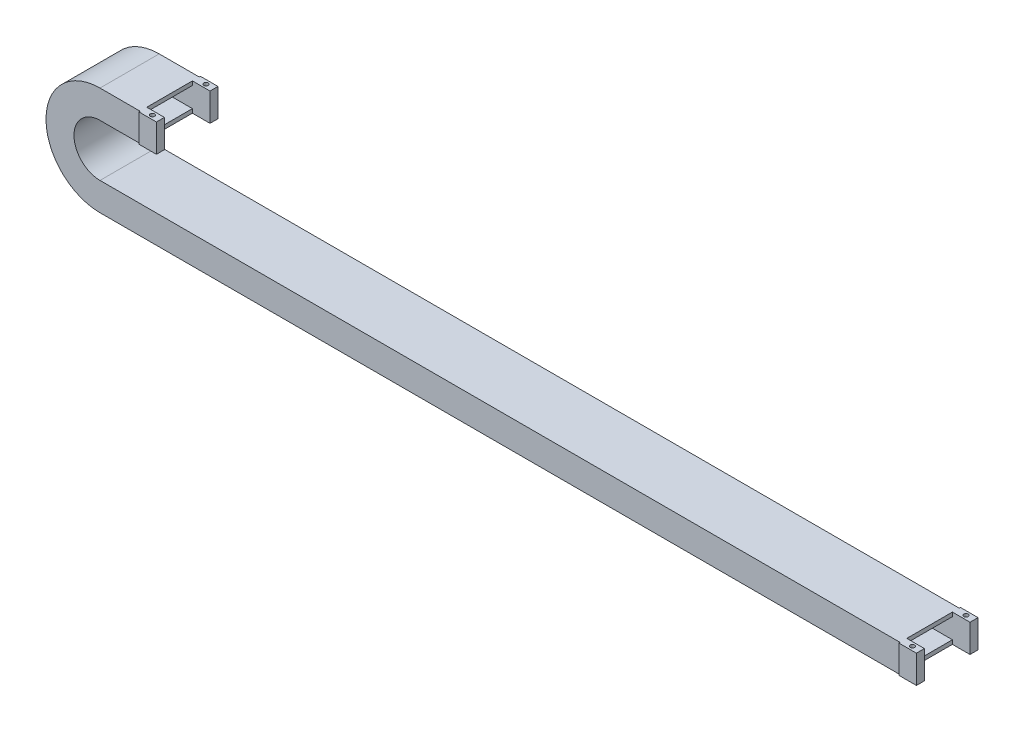
SolidWorks part; units mm, degrees
ref_plane "前视基准面" through (0, 0, 0) normal (0, 0, 1) x (1, 0, 0)
ref_plane "上视基准面" through (0, 0, 0) normal (0, 1, 0) x (1, 0, 0)
ref_plane "右视基准面" through (0, 0, 0) normal (1, 0, 0) x (0, 0, -1)
sketch "草图1" plane through (0, 0, 0) normal (0, 0, 1) x (1, 0, 0)
  line L0 (0, 0) -> (-1000, 0)
  line L1 (-1000, 100) -> (-950, 100)
  arc A0 (-1000, 100) -> (-1000, 0) centre (-1000, 50) ccw
  dimension "D2" = 50
  dimension "D1" = 1000
  dimension "D3" = 50
sketch "草图2" plane through (0, 0, 0) normal (1, 0, 0) x (0, 0, -1)
  line L1 (37, 17.5) -> (-37, 17.5)
  line L2 (37, 17.5) -> (37, -17.5)
  line L3 (37, -17.5) -> (-37, -17.5)
  line L4 (-37, 17.5) -> (-37, -17.5)
  line L5 (37, 17.5) -> (-37, -17.5) construction
  line L6 (37, -17.5) -> (-37, 17.5) construction
  line L7 (28.5, 12.5) -> (-28.5, 12.5)
  line L8 (28.5, 12.5) -> (28.5, -12.5)
  line L9 (28.5, -12.5) -> (-28.5, -12.5)
  line L10 (-28.5, 12.5) -> (-28.5, -12.5)
  line L11 (28.5, 12.5) -> (-28.5, -12.5) construction
  line L12 (28.5, -12.5) -> (-28.5, 12.5) construction
  point P0 (0, 0)
  point P5 (0, 0)
  dimension "D1" = 35
  dimension "D2" = 74
  dimension "D3" = 25
  dimension "D4" = 57
sweep "扫描1" add profiles "草图2" path "草图1"
shell "抽壳1" [suppressed] thickness 3
sketch "草图11" plane through (0, 0, 0) normal (1, 0, 0) x (0, 0, -1)
  line L0 (37, 17.5) -> (-37, 17.5) construction
  line L1 (-38.5, 17.5) -> (38.5, 17.5)
  line L2 (-38.5, 17.5) -> (-38.5, -17.5)
  line L3 (-38.5, -17.5) -> (38.5, -17.5)
  line L4 (38.5, 17.5) -> (38.5, -17.5)
  line L5 (-38.5, 17.5) -> (38.5, -17.5) construction
  line L6 (-38.5, -17.5) -> (38.5, 17.5) construction
  line L7 (-28.5, -12.5) -> (28.5, -12.5) construction
  line L8 (28.5, -12.5) -> (28.5, 12.5) construction
  line L9 (28.5, 12.5) -> (-28.5, 12.5) construction
  line L10 (-28.5, 12.5) -> (-28.5, -12.5) construction
  line L11 (-28.5, -12.5) -> (28.5, -12.5)
  line L12 (28.5, -12.5) -> (28.5, 12.5)
  line L13 (28.5, 12.5) -> (-28.5, 12.5)
  line L14 (-28.5, 12.5) -> (-28.5, -12.5)
  point P0 (0, 0)
  dimension "D1" = 77
extrude "凸台-拉伸1" add sketch "草图11" along normal blind 22
sketch "草图12" plane through (0, 17.5, 0) normal (0, 1, 0) x (1, 0, 0)
  line L0 (22, 38.5) -> (22, -38.5) construction
  line L1 (0, 28.5) -> (23.0119, 28.5)
  line L2 (0, 28.5) -> (0, -28.5)
  line L3 (0, -28.5) -> (23.0119, -28.5)
  line L4 (23.0119, 28.5) -> (23.0119, -28.5)
  line L5 (0, 28.5) -> (23.0119, -28.5) construction
  line L6 (0, -28.5) -> (23.0119, 28.5) construction
  point P0 (11.506, 0)
  dimension "D1" = 57
  dimension "D2" = 22
extrude "切除-拉伸9" cut sketch "草图12" against normal through all
hole_wizard "Ø5.5 (5.5) 直径孔1" positions "草图14" profile "草图13" hole size "Ø5.5" standard "GB" end condition through all
sketch "草图14" plane through (0, 17.5, 0) normal (0, 1, 0) x (1, 0, 0)
  line L0 (12, 33.5) -> (12, -33.5) construction
  line L3 (0, 0) -> (12, 0) construction
  line L6 (22, 38.5) -> (22, 28.5) construction
  point P0 (12, 33.5)
  point P2 (12, -33.5)
  dimension "D1" = 67
  dimension "D2" = 10
sketch "草图13" plane through (12, 17.5, -33.5) normal (1, 0, 0) x (0, 0, 1)
  line L0 (0, 0) -> (0, 35.0001)
  line L1 (0, 35.0001) -> (2.75, 35.0001)
  line L2 (2.75, 35.0001) -> (2.75, 0)
  line L5 (2.75, 0) -> (0, 0)
  line L11 (0, -6.35) -> (0, 107.95) construction
  dimension "通孔孔直径" = 5.5
  dimension "通孔孔深度" = 35.0001
sketch "草图15" plane through (-950, 0, 0) normal (1, 0, 0) x (0, 0, -1)
  line L0 (0, 100) -> (0, 0) construction
  line L1 (-38.5, 117.5) -> (38.5, 117.5)
  line L2 (-38.5, 117.5) -> (-38.5, 82.5)
  line L3 (-38.5, 82.5) -> (38.5, 82.5)
  line L4 (38.5, 117.5) -> (38.5, 82.5)
  line L5 (-38.5, 117.5) -> (38.5, 82.5) construction
  line L6 (-38.5, 82.5) -> (38.5, 117.5) construction
  line L7 (-37, 117.5) -> (37, 117.5) construction
  line L8 (37, 82.5) -> (-37, 82.5) construction
  line L9 (28.5, 112.5) -> (28.5, 87.5) construction
  line L10 (28.5, 87.5) -> (-28.5, 87.5) construction
  line L11 (-28.5, 112.5) -> (28.5, 112.5) construction
  line L12 (-28.5, 87.5) -> (-28.5, 112.5) construction
  line L13 (28.5, 112.5) -> (28.5, 87.5)
  line L14 (28.5, 87.5) -> (-28.5, 87.5)
  line L15 (-28.5, 112.5) -> (28.5, 112.5)
  line L16 (-28.5, 87.5) -> (-28.5, 112.5)
  line L17 (-38.5, 17.5) -> (38.5, 17.5) construction
  point P0 (0, 100)
extrude "凸台-拉伸2" add sketch "草图15" along normal blind 22
sketch "草图16" plane through (0, 117.5, 0) normal (0, 1, 0) x (1, 0, 0)
  line L0 (0, 0) -> (-1000, 0) construction
  line L1 (-950, 28.5) -> (-904.2045, 28.5)
  line L2 (-950, 28.5) -> (-950, -28.5)
  line L3 (-950, -28.5) -> (-904.2045, -28.5)
  line L4 (-904.2045, 28.5) -> (-904.2045, -28.5)
  line L5 (-950, 28.5) -> (-904.2045, -28.5) construction
  line L6 (-950, -28.5) -> (-904.2045, 28.5) construction
  line L7 (-927.1023, 0) -> (-928, 0) construction
  line L8 (-928, 38.5) -> (-928, -38.5) construction
  point P0 (-927.1023, 0)
  dimension "D1" = 57
  dimension "D2" = 22
extrude "切除-拉伸10" cut sketch "草图16" against normal blind 49
hole_wizard "Ø5.5 (5.5) 直径孔2" positions "草图18" profile "草图17" hole size "Ø5.5" standard "GB"
sketch "草图18" plane through (0, 117.5, 0) normal (0, 1, 0) x (1, 0, 0)
  line L0 (-938, 33.5) -> (-938, -33.5) construction
  line L3 (-950, 0) -> (-938, 0) construction
  line L4 (-950, 28.5) -> (-950, -28.5) construction
  line L7 (-928, 38.5) -> (-928, 28.5) construction
  line L8 (12, 33.5) -> (12, -33.5) construction
  point P0 (-938, 33.5)
  point P2 (-938, -33.5)
  dimension "D2" = 10
sketch "草图17" plane through (-938, 117.5, -33.5) normal (1, 0, 0) x (0, 0, 1)
  line L0 (0, 0) -> (0, 51.6524)
  line L1 (0, 51.6524) -> (2.75, 50)
  line L2 (2.75, 50) -> (2.75, 0)
  line L5 (2.75, 0) -> (0, 0)
  line L10 (0, 51.6524) -> (-2.75, 50) construction
  line L11 (0, -6.35) -> (0, 107.95) construction
  dimension "孔直径" = 5.5
  dimension "孔深度" = 50
  dimension "导头角度" = 118
